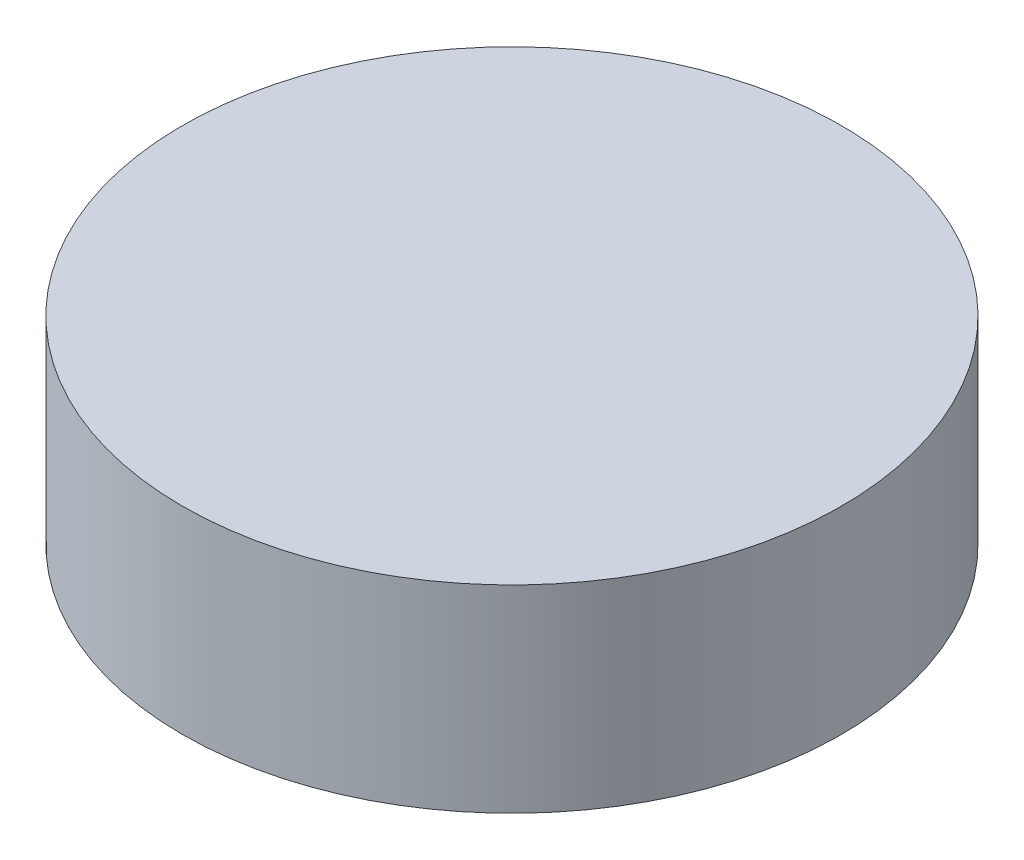
SolidWorks part; units mm, degrees
ref_plane "Front Plane" through (0, 0, 0) normal (0, 0, 1) x (1, 0, 0)
ref_plane "Top Plane" through (0, 0, 0) normal (0, 1, 0) x (1, 0, 0)
ref_plane "Right Plane" through (0, 0, 0) normal (1, 0, 0) x (0, 0, -1)
sketch "Sketch1" plane through (0, 0, 0) normal (0, 1, 0) x (1, 0, 0)
  circle A1 centre (0, 0) radius 10
  dimension "D1" = 20
extrude "Boss-Extrude1" add sketch "Sketch1" along normal blind 6
